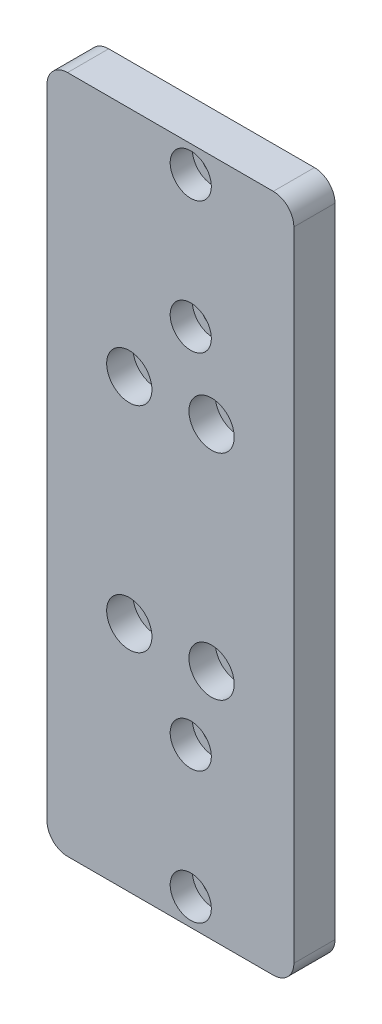
from build123d import *

# Parameters (mm, degrees)
SKETCH1_W                                           = 60
SKETCH1_H                                           = 165
BOSS_EXTRUDE1_DEPTH                                 = 10
CBORE_FOR_M6_HEX_SOCKET_HEAD_CAP_SCREW1_D           = 6.6
CBORE_FOR_M6_HEX_SOCKET_HEAD_CAP_SCREW1_CBORE_D     = 11
CBORE_FOR_M6_HEX_SOCKET_HEAD_CAP_SCREW1_CBORE_DEPTH = 6.4
CBORE_FOR_M5_HEX_SOCKET_HEAD_CAP_SCREW2_D           = 5.5
CBORE_FOR_M5_HEX_SOCKET_HEAD_CAP_SCREW2_CBORE_D     = 10
CBORE_FOR_M5_HEX_SOCKET_HEAD_CAP_SCREW2_CBORE_DEPTH = 5.4
FILLET1_R                                           = 5


with BuildPart() as part:
    # Sketch1 → Boss-Extrude1 (new body)
    with BuildSketch(Plane.XY):
        Rectangle(SKETCH1_W, SKETCH1_H)
    extrude(amount=BOSS_EXTRUDE1_DEPTH)

    # CBORE for M6 Hex Socket Head Cap Screw1 (through all)
    with Locations(Plane.XY.offset(10)):
        with Locations((-10, 26), (10, 26), (10, -26), (-10, -26)):
            CounterBoreHole(CBORE_FOR_M6_HEX_SOCKET_HEAD_CAP_SCREW1_D / 2, CBORE_FOR_M6_HEX_SOCKET_HEAD_CAP_SCREW1_CBORE_D / 2, CBORE_FOR_M6_HEX_SOCKET_HEAD_CAP_SCREW1_CBORE_DEPTH)

    # CBORE for M5 Hex Socket Head Cap Screw2 (through all)
    with Locations(Plane.XY.offset(10)):
        with Locations((4.94295756, 76), (4.94295756, 44), (4.94295756, -44), (4.94295756, -76)):
            CounterBoreHole(CBORE_FOR_M5_HEX_SOCKET_HEAD_CAP_SCREW2_D / 2, CBORE_FOR_M5_HEX_SOCKET_HEAD_CAP_SCREW2_CBORE_D / 2, CBORE_FOR_M5_HEX_SOCKET_HEAD_CAP_SCREW2_CBORE_DEPTH)

    # Fillet1
    fillet1_edges = [part.edges().sort_by_distance(p)[0] for p in [
        (30, -82.5, 5),
        (-30, -82.5, 5),
        (-30, 82.5, 5),
        (30, 82.5, 5),
    ]]
    fillet(fillet1_edges, radius=FILLET1_R)


solid = part.part
